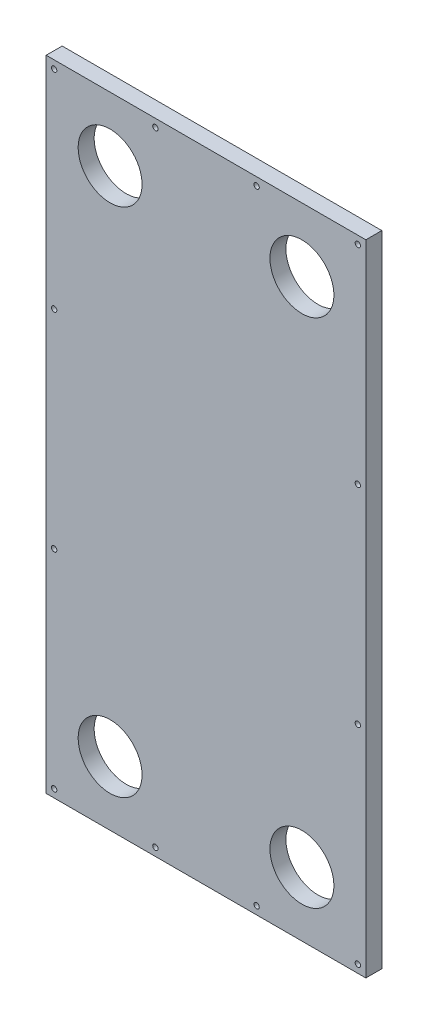
from build123d import *

# Parameters (mm, degrees)
SKETCH1_W                 = 600
SKETCH1_H                 = 1200
BOSS_EXTRUDE1_DEPTH       = 30
SKETCH2_R                 = 60
CUT_EXTRUDE1_DEPTH        = 42
SKETCH3_R                 = 5
CUT_EXTRUDE2_DEPTH        = 40
LPATTERN1_COUNT           = 4
LPATTERN1_PITCH           = 390
LPATTERN2_COUNT           = 2
LPATTERN2_PITCH           = 570
LPATTERN2_COPY_1_SKETCH_R = 5
LPATTERN2_COPY_1_DEPTH    = 40
LPATTERN2_COPY_2_SKETCH_R = 5
LPATTERN2_COPY_2_DEPTH    = 40
LPATTERN2_COPY_3_SKETCH_R = 5
LPATTERN2_COPY_3_DEPTH    = 40
LPATTERN3_COUNT           = 3
LPATTERN3_PITCH           = 190
LPATTERN4_COPY_1_SKETCH_R = 5
LPATTERN4_COPY_1_DEPTH    = 40
LPATTERN4_COPY_2_SKETCH_R = 5
LPATTERN4_COPY_2_DEPTH    = 40
LPATTERN4_COPY_3_SKETCH_R = 5
LPATTERN4_COPY_3_DEPTH    = 40
SKETCH4_R                 = 10
CUT_EXTRUDE3_DEPTH        = 15
LPATTERN5_COUNT           = 4
LPATTERN5_PITCH           = 390
LPATTERN6_COUNT           = 2
LPATTERN6_PITCH           = 570
LPATTERN6_COPY_1_SKETCH_R = 10
LPATTERN6_COPY_1_DEPTH    = 15
LPATTERN6_COPY_2_SKETCH_R = 10
LPATTERN6_COPY_2_DEPTH    = 15
LPATTERN6_COPY_3_SKETCH_R = 10
LPATTERN6_COPY_3_DEPTH    = 15
LPATTERN8_COUNT           = 3
LPATTERN8_PITCH           = 190
LPATTERN9_COPY_1_SKETCH_R = 10
LPATTERN9_COPY_1_DEPTH    = 15
LPATTERN9_COPY_2_SKETCH_R = 10
LPATTERN9_COPY_2_DEPTH    = 15
LPATTERN9_COPY_3_SKETCH_R = 10
LPATTERN9_COPY_3_DEPTH    = 15


with BuildPart() as part:
    # Sketch1 → Boss-Extrude1 (new body)
    with BuildSketch(Plane.XY):
        Rectangle(SKETCH1_W, SKETCH1_H)
    extrude(amount=BOSS_EXTRUDE1_DEPTH)

    # Sketch2 → Cut-Extrude1 (cut)
    with BuildSketch(Plane(origin=(0, 0, 0), x_dir=(-1, 0, 0), z_dir=(0, 0, -1))):
        with Locations((-180, 480)):
            Circle(SKETCH2_R)
        with Locations((180, 480)):
            Circle(SKETCH2_R)
        with Locations((180, -480)):
            Circle(SKETCH2_R)
        with Locations((-180, -480)):
            Circle(SKETCH2_R)
    extrude(amount=-CUT_EXTRUDE1_DEPTH, mode=Mode.SUBTRACT)

    # Sketch3 → Cut-Extrude2 (cut)
    with BuildSketch(Plane(origin=(0, 0, 0), x_dir=(-1, 0, 0), z_dir=(0, 0, -1))):
        with Locations((-285, 585)):
            Circle(SKETCH3_R)
    cut_extrude2 = extrude(amount=-CUT_EXTRUDE2_DEPTH, mode=Mode.SUBTRACT)

    # LPattern1: Cut-Extrude2 ×4
    with Locations(*[(0, -i * LPATTERN1_PITCH, 0) for i in range(1, LPATTERN1_COUNT)]):
        add(cut_extrude2, mode=Mode.SUBTRACT)

    # LPattern2: Cut-Extrude2 ×2
    with Locations(*[(-i * LPATTERN2_PITCH, 0, 0) for i in range(1, LPATTERN2_COUNT)]):
        add(cut_extrude2, mode=Mode.SUBTRACT)

    # LPattern2 copy 1 sketch → LPattern2 copy 1 (cut)
    with BuildSketch(Plane(origin=(-570, -390, 0), x_dir=(-1, 0, 0), z_dir=(0, 0, -1))):
        with Locations((-285, 585)):
            Circle(LPATTERN2_COPY_1_SKETCH_R)
    extrude(amount=-LPATTERN2_COPY_1_DEPTH, mode=Mode.SUBTRACT)

    # LPattern2 copy 2 sketch → LPattern2 copy 2 (cut)
    with BuildSketch(Plane(origin=(-570, -780, 0), x_dir=(-1, 0, 0), z_dir=(0, 0, -1))):
        with Locations((-285, 585)):
            Circle(LPATTERN2_COPY_2_SKETCH_R)
    extrude(amount=-LPATTERN2_COPY_2_DEPTH, mode=Mode.SUBTRACT)

    # LPattern2 copy 3 sketch → LPattern2 copy 3 (cut)
    with BuildSketch(Plane(origin=(-570, -1170, 0), x_dir=(-1, 0, 0), z_dir=(0, 0, -1))):
        with Locations((-285, 585)):
            Circle(LPATTERN2_COPY_3_SKETCH_R)
    extrude(amount=-LPATTERN2_COPY_3_DEPTH, mode=Mode.SUBTRACT)

    # LPattern3: Cut-Extrude2 ×3
    with Locations(*[(-i * LPATTERN3_PITCH, 0, 0) for i in range(1, LPATTERN3_COUNT)]):
        add(cut_extrude2, mode=Mode.SUBTRACT)

    # LPattern4 copy 1 sketch → LPattern4 copy 1 (cut)
    with BuildSketch(Plane(origin=(-190, -1170, 0), x_dir=(-1, 0, 0), z_dir=(0, 0, -1))):
        with Locations((-285, 585)):
            Circle(LPATTERN4_COPY_1_SKETCH_R)
    extrude(amount=-LPATTERN4_COPY_1_DEPTH, mode=Mode.SUBTRACT)

    # LPattern4 copy 2 sketch → LPattern4 copy 2 (cut)
    with BuildSketch(Plane(origin=(-380, -1170, 0), x_dir=(-1, 0, 0), z_dir=(0, 0, -1))):
        with Locations((-285, 585)):
            Circle(LPATTERN4_COPY_2_SKETCH_R)
    extrude(amount=-LPATTERN4_COPY_2_DEPTH, mode=Mode.SUBTRACT)

    # LPattern4 copy 3 sketch → LPattern4 copy 3 (cut)
    with BuildSketch(Plane(origin=(0, -1170, 0), x_dir=(-1, 0, 0), z_dir=(0, 0, -1))):
        with Locations((-285, 585)):
            Circle(LPATTERN4_COPY_3_SKETCH_R)
    extrude(amount=-LPATTERN4_COPY_3_DEPTH, mode=Mode.SUBTRACT)

    # Sketch4 → Cut-Extrude3 (cut)
    with BuildSketch(Plane(origin=(0, 0, 0), x_dir=(-1, 0, 0), z_dir=(0, 0, -1))):
        with Locations((-285, 585)):
            Circle(SKETCH4_R)
    cut_extrude3 = extrude(amount=-CUT_EXTRUDE3_DEPTH, mode=Mode.SUBTRACT)

    # LPattern5: Cut-Extrude3 ×4
    with Locations(*[(0, -i * LPATTERN5_PITCH, 0) for i in range(1, LPATTERN5_COUNT)]):
        add(cut_extrude3, mode=Mode.SUBTRACT)

    # LPattern6: Cut-Extrude3 ×2
    with Locations(*[(-i * LPATTERN6_PITCH, 0, 0) for i in range(1, LPATTERN6_COUNT)]):
        add(cut_extrude3, mode=Mode.SUBTRACT)

    # LPattern6 copy 1 sketch → LPattern6 copy 1 (cut)
    with BuildSketch(Plane(origin=(-570, -390, 0), x_dir=(-1, 0, 0), z_dir=(0, 0, -1))):
        with Locations((-285, 585)):
            Circle(LPATTERN6_COPY_1_SKETCH_R)
    extrude(amount=-LPATTERN6_COPY_1_DEPTH, mode=Mode.SUBTRACT)

    # LPattern6 copy 2 sketch → LPattern6 copy 2 (cut)
    with BuildSketch(Plane(origin=(-570, -780, 0), x_dir=(-1, 0, 0), z_dir=(0, 0, -1))):
        with Locations((-285, 585)):
            Circle(LPATTERN6_COPY_2_SKETCH_R)
    extrude(amount=-LPATTERN6_COPY_2_DEPTH, mode=Mode.SUBTRACT)

    # LPattern6 copy 3 sketch → LPattern6 copy 3 (cut)
    with BuildSketch(Plane(origin=(-570, -1170, 0), x_dir=(-1, 0, 0), z_dir=(0, 0, -1))):
        with Locations((-285, 585)):
            Circle(LPATTERN6_COPY_3_SKETCH_R)
    extrude(amount=-LPATTERN6_COPY_3_DEPTH, mode=Mode.SUBTRACT)

    # LPattern8: Cut-Extrude3 ×3
    with Locations(*[(-i * LPATTERN8_PITCH, 0, 0) for i in range(1, LPATTERN8_COUNT)]):
        add(cut_extrude3, mode=Mode.SUBTRACT)

    # LPattern9 copy 1 sketch → LPattern9 copy 1 (cut)
    with BuildSketch(Plane(origin=(-190, -1170, 0), x_dir=(-1, 0, 0), z_dir=(0, 0, -1))):
        with Locations((-285, 585)):
            Circle(LPATTERN9_COPY_1_SKETCH_R)
    extrude(amount=-LPATTERN9_COPY_1_DEPTH, mode=Mode.SUBTRACT)

    # LPattern9 copy 2 sketch → LPattern9 copy 2 (cut)
    with BuildSketch(Plane(origin=(-380, -1170, 0), x_dir=(-1, 0, 0), z_dir=(0, 0, -1))):
        with Locations((-285, 585)):
            Circle(LPATTERN9_COPY_2_SKETCH_R)
    extrude(amount=-LPATTERN9_COPY_2_DEPTH, mode=Mode.SUBTRACT)

    # LPattern9 copy 3 sketch → LPattern9 copy 3 (cut)
    with BuildSketch(Plane(origin=(0, -1170, 0), x_dir=(-1, 0, 0), z_dir=(0, 0, -1))):
        with Locations((-285, 585)):
            Circle(LPATTERN9_COPY_3_SKETCH_R)
    extrude(amount=-LPATTERN9_COPY_3_DEPTH, mode=Mode.SUBTRACT)


solid = part.part
